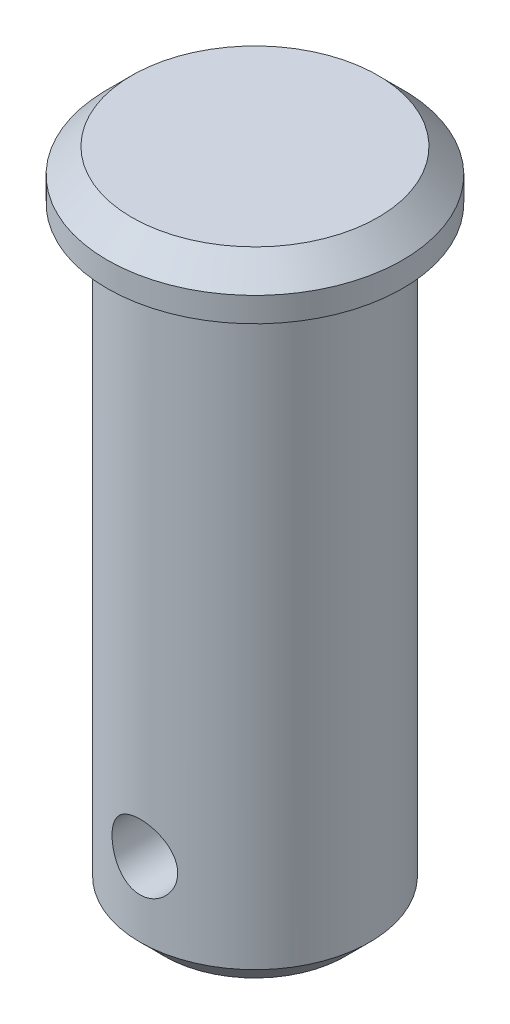
SolidWorks part; units mm, degrees
material "45"
ref_plane "前视基准面" through (0, 0, 0) normal (0, 0, 1) x (1, 0, 0)
ref_plane "上视基准面" through (0, 0, 0) normal (0, 1, 0) x (1, 0, 0)
ref_plane "右视基准面" through (0, 0, 0) normal (1, 0, 0) x (0, 0, -1)
sketch "草图1" plane through (0, 0, 0) normal (0, 1, 0) x (1, 0, 0)
  circle A0 centre (0, 0) radius 9
  dimension "D1" = 18
extrude "凸台-拉伸1" add sketch "草图1" along normal blind 3
sketch "草图2" plane through (0, 0, 0) normal (0, -1, 0) x (1, 0, 0)
  circle A0 centre (0, 0) radius 7
  dimension "D1" = 14
extrude "凸台-拉伸2" add sketch "草图2" along normal blind 37
ref_plane "基准面1" through (-7, 0, 0) normal (-1, 0, 0) x (0, 0, 1)
chamfer "倒角1" distance 1.5 angle 45 2 edges at (0, -37, -7) (0, 3, 9)
sketch "草图10" plane through (0, 0, 0) normal (0, 0, 1) x (1, 0, 0)
  line L0 (-5.5, -37) -> (5.5, -37) construction
  circle A0 centre (0, -31) radius 2
  dimension "D1" = 4
  dimension "D2" = 6
extrude "切除-拉伸2" cut sketch "草图10" against normal through all both and the other way through all
fillet "圆角1" radius 0.5 1 edges at (0, 0, -7)
